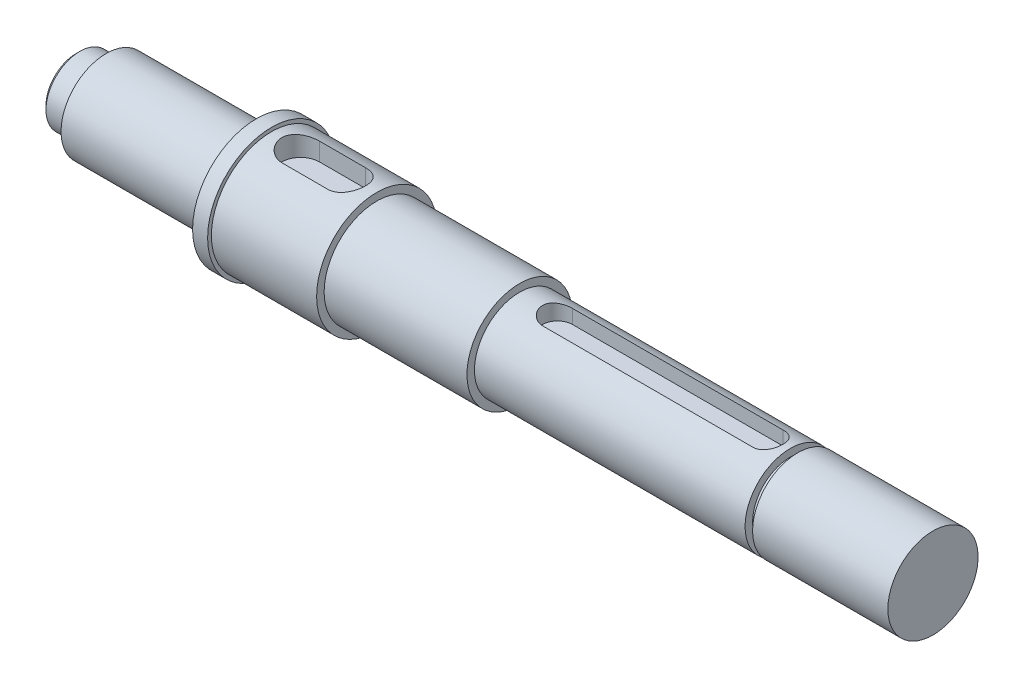
from build123d import *

# Parameters (mm, degrees)
CUT_EXTRUDE_1_DEPTH = 2.2
CUT_EXTRUDE_2_DEPTH = 2.8


with BuildPart() as part:
    # 草图1 → 旋转1 (revolve)
    with BuildSketch(Plane.XY, mode=Mode.PRIVATE) as revolve_1_sk:
        Polygon((-46.103902345, 8.5), (-44.103902345, 8.5), (-44.103902345, 8), (-30.103902345, 8), (-30.103902345, 7), (-11.103902345, 7), (-11.103902345, 6), (24.896097655, 6), (24.896097655, 5), (25.896097655, 5), (25.896097655, 6), (43.896097655, 6), (43.896097655, 0), (-70.103902345, 0), (-70.103902345, 4), (-69.603902345, 4.5), (-66.103902345, 4.5), (-66.103902345, 6), (-46.103902345, 6), align=None)
    revolve(revolve_1_sk.sketch.rotate(Axis((-70.103902345, 0, 0), (1, 0, 0)), 90), axis=Axis((-70.103902345, 0, 0), (1, 0, 0)))

    # 草图7 → 切除-拉伸1 (cut)
    with BuildSketch(Plane(origin=(0, 6, 0), x_dir=(1, 0, 0), z_dir=(0, 1, 0))):
        with BuildLine():
            Line((-6.053902345, 2), (21.946097655, 2))
            ThreePointArc((21.946097655, 2), (23.946097655, 0), (21.946097655, -2))
            Line((21.946097655, -2), (-6.053902345, -2))
            ThreePointArc((-6.053902345, -2), (-8.053902345, 0), (-6.053902345, 2))
        make_face()
    extrude(amount=-CUT_EXTRUDE_1_DEPTH, mode=Mode.SUBTRACT)

    # 草图9 → 切除-拉伸2 (cut)
    with BuildSketch(Plane(origin=(0, 8, 0), x_dir=(1, 0, 0), z_dir=(0, 1, 0))):
        with BuildLine():
            Line((-40.225350305, 2.5), (-34.103902345, 2.5))
            ThreePointArc((-34.103902345, 2.5), (-31.603902345, 0), (-34.103902345, -2.5))
            Line((-34.103902345, -2.5), (-40.225350305, -2.5))
            ThreePointArc((-40.225350305, -2.5), (-42.725350305, 0), (-40.225350305, 2.5))
        make_face()
    extrude(amount=-CUT_EXTRUDE_2_DEPTH, mode=Mode.SUBTRACT)


solid = part.part
